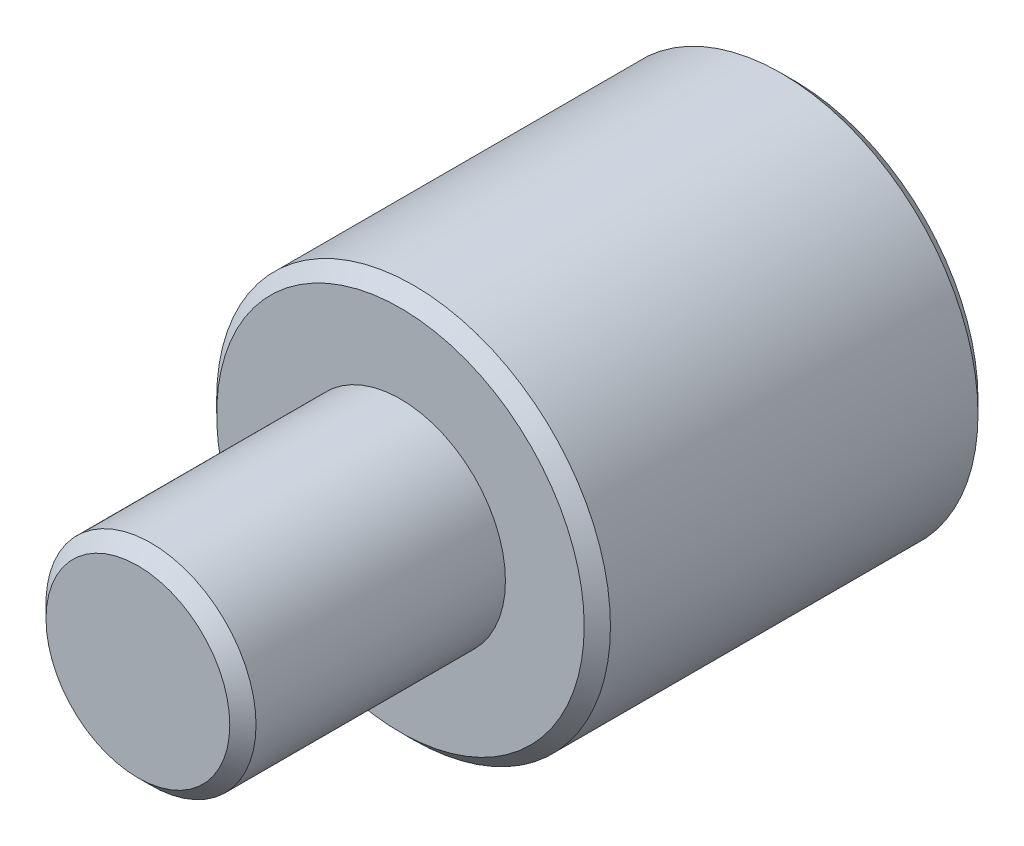
from build123d import *

# Parameters (mm, degrees)
SKETCH1_R           = 7.5
BOSS_EXTRUDE1_DEPTH = 15
SKETCH2_R           = 4
BOSS_EXTRUDE2_DEPTH = 10
CHAMFER1_SIZE       = 0.5


with BuildPart() as part:
    # Sketch1 → Boss-Extrude1 (new body)
    with BuildSketch(Plane.XY):
        Circle(SKETCH1_R)
    extrude(amount=BOSS_EXTRUDE1_DEPTH)

    # Sketch2 → Boss-Extrude2 (add)
    with BuildSketch(Plane.XY.offset(15)):
        Circle(SKETCH2_R)
    extrude(amount=BOSS_EXTRUDE2_DEPTH)

    # Chamfer1
    chamfer1_edges = [part.edges().sort_by_distance(p)[0] for p in [
        (-7.5, 0, 0),
        (-7.5, 0, 15),
        (-4, 0, 25),
    ]]
    chamfer(chamfer1_edges, length=CHAMFER1_SIZE)


solid = part.part
